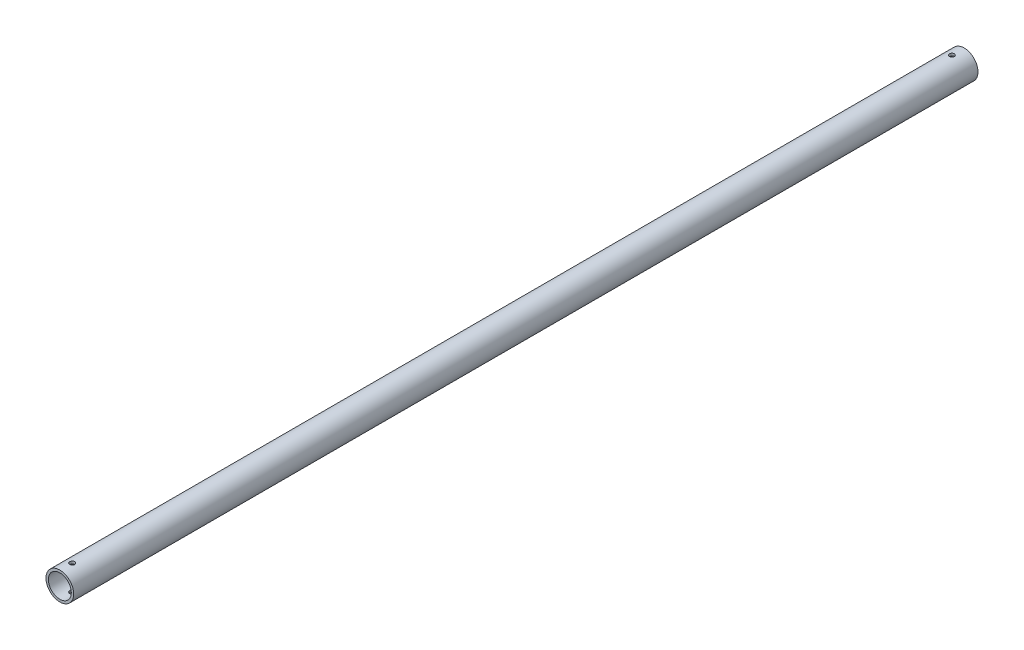
SolidWorks part; units mm, degrees
material "1023 碳钢板 (SS)"
ref_plane "前视基准面" through (0, 0, 0) normal (0, 0, 1) x (1, 0, 0)
ref_plane "上视基准面" through (0, 0, 0) normal (0, 1, 0) x (1, 0, 0)
ref_plane "右视基准面" through (0, 0, 0) normal (1, 0, 0) x (0, 0, -1)
sketch "草图1" plane through (0, 0, 0) normal (0, 0, 1) x (1, 0, 0)
  circle A0 centre (0, 0) radius 16.85
  circle A1 centre (0, 0) radius 13.95
  dimension "D1" = 33.7
  dimension "D2" = 27.9
extrude "凸台-拉伸1" add sketch "草图1" along normal blind 1100
sketch "草图2" plane through (0, 0, 0) normal (0, 1, 0) x (1, 0, 0)
  line L0 (13.95, 0) -> (-13.95, 0) construction
  line L1 (-16.85, -1100) -> (16.85, -1100) construction
  circle A0 centre (0, -15) radius 3
  circle A1 centre (0, -1085) radius 3
  dimension "D1" = 6
  dimension "D2" = 6
  dimension "D3" = 15
  dimension "D4" = 15
extrude "切除-拉伸1" cut sketch "草图2" against normal mid plane 33.7
